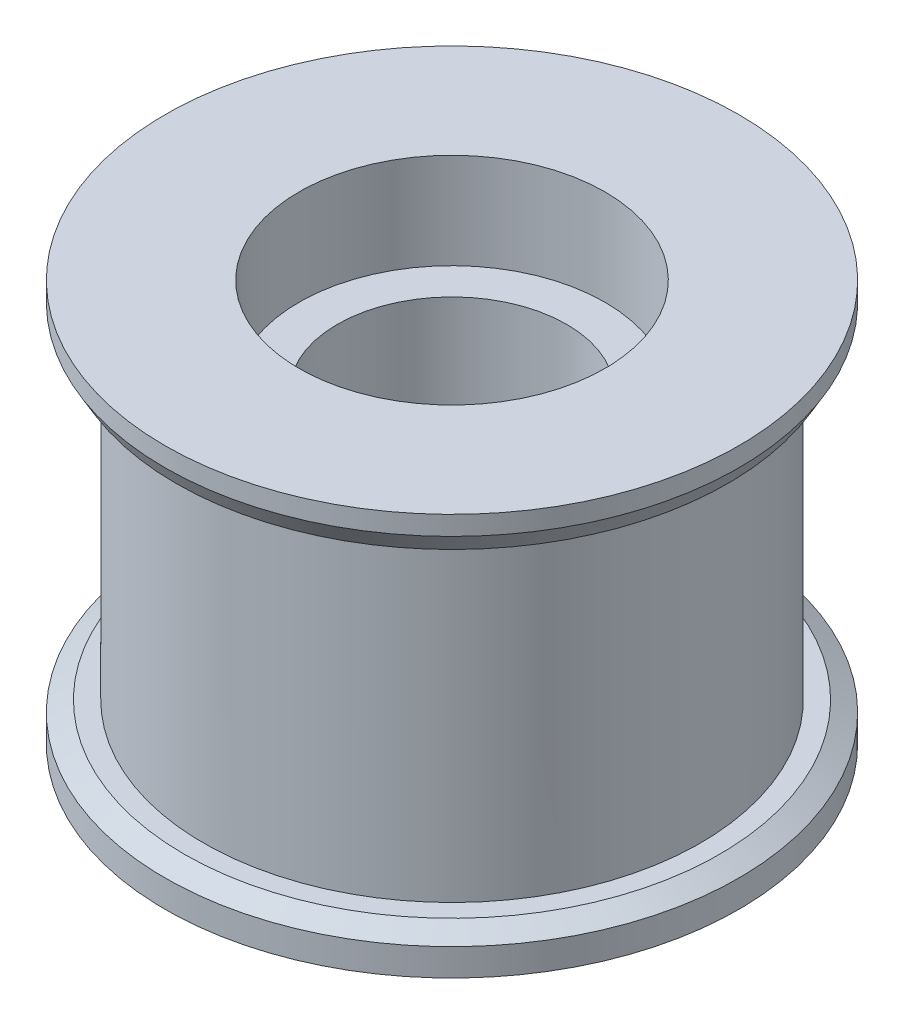
from build123d import *

# Parameters (mm, degrees)
SKETCH_1_W          = 6.99
SKETCH_1_H          = 21
SKETCH_4_R          = 8
CUT_EXTRUDE_3_DEPTH = 5
SKETCH_5_R          = 15
SKETCH_5_R_2        = 8
EXTRUDE_1_DEPTH     = 2
CHAMFER_1_SIZE      = 1
CHAMFER_1_SIZE2     = 0.577350269
CHAMFER_2_SIZE      = 1
CHAMFER_2_SIZE2     = 0.577350269


with BuildPart() as part:
    # 草图1 → 旋转1 (revolve)
    with BuildSketch(Plane.XY, mode=Mode.PRIVATE) as revolve_1_sk:
        with Locations((9.495, 0)):
            Rectangle(SKETCH_1_W, SKETCH_1_H)
    revolve(revolve_1_sk.sketch.rotate(Axis((0, 0, 0), (0, 1, 0)), 90), axis=Axis((0, 0, 0), (0, 1, 0)))

    # 草图4 → 切除-拉伸3 (cut)
    with BuildSketch(Plane.XZ.offset(10.5)):
        with Locations(Location((0, 0, 0), (0, 0, 270))):
            Circle(SKETCH_4_R)
    cut_extrude_3 = extrude(amount=-CUT_EXTRUDE_3_DEPTH, mode=Mode.SUBTRACT)

    # 草图5 → 凸台-拉伸1 (add)
    with BuildSketch(Plane.XZ.offset(10.5)):
        with Locations(Location((0, 0, 0), (0, 0, 270))):
            Circle(SKETCH_5_R)
        with Locations(Location((0, 0, 0), (0, 0, 270))):
            Circle(SKETCH_5_R_2, mode=Mode.SUBTRACT)
    extrude_1 = extrude(amount=-EXTRUDE_1_DEPTH)

    # 镜向1: 切除-拉伸3, 凸台-拉伸1 across plane
    add(cut_extrude_3.mirror(Plane.ZX), mode=Mode.SUBTRACT)
    add(extrude_1.mirror(Plane.ZX))

    # 倒角1
    chamfer_1_edges = [part.edges().sort_by_distance(p)[0] for p in [
        (0, 8.5, 15),
    ]]
    chamfer_1_side = [part.faces().sort_by_distance(p)[0] for p in [
        (0, 9.5, 15),
    ]]
    chamfer(chamfer_1_edges, length=CHAMFER_1_SIZE, length2=CHAMFER_1_SIZE2, reference=chamfer_1_side[0])

    # 倒角2
    chamfer_2_edges = [part.edges().sort_by_distance(p)[0] for p in [
        (0, -8.5, 15),
    ]]
    chamfer_2_side = [part.faces().sort_by_distance(p)[0] for p in [
        (0, -8.5, 14.575735931),
    ]]
    chamfer(chamfer_2_edges, length=CHAMFER_2_SIZE, length2=CHAMFER_2_SIZE2, reference=chamfer_2_side[0])


solid = part.part
